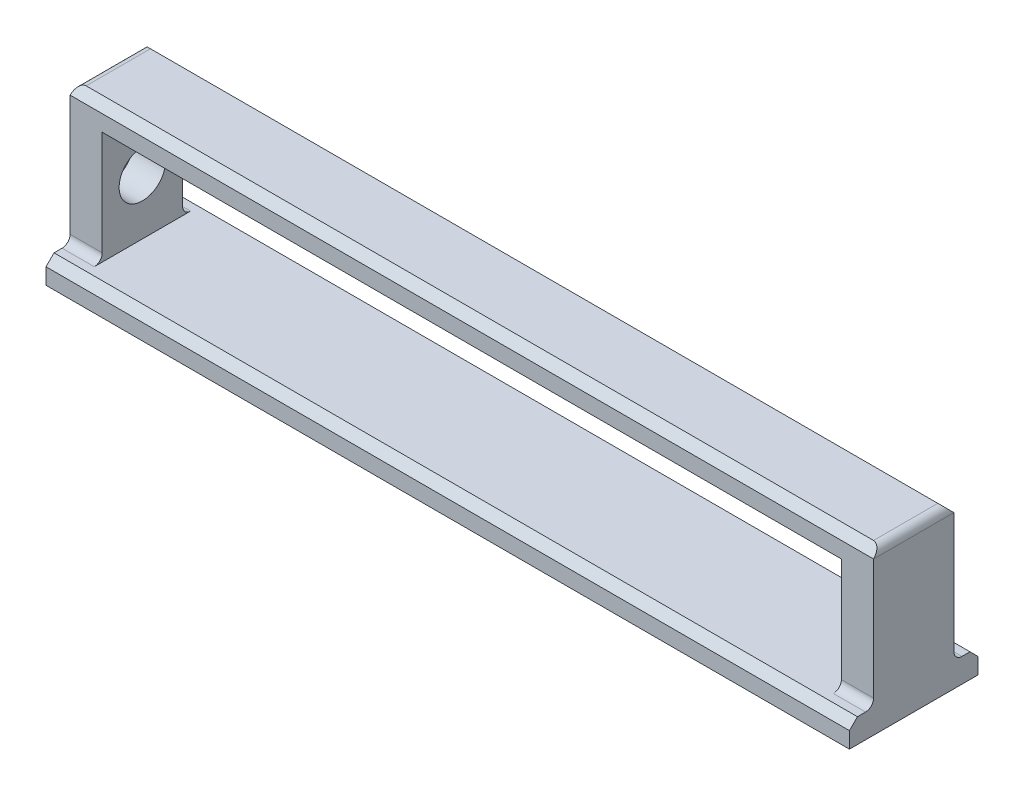
SolidWorks part; units mm, degrees
material "铸造碳钢"
ref_plane "Front Plane" through (0, 0, 0) normal (0, 0, 1) x (1, 0, 0)
ref_plane "Top Plane" through (0, 0, 0) normal (0, 1, 0) x (1, 0, 0)
ref_plane "Right Plane" through (0, 0, 0) normal (1, 0, 0) x (0, 0, -1)
sketch "Sketch1" plane through (0, 0, 0) normal (0, 0, 1) x (1, 0, 0)
  line L0 (0, 1000) -> (5000, 1000)
  line L3 (5000, 0) -> (0, 0)
  line L4 (5000, 1000) -> (5000, 0)
  line L11 (0, 1000) -> (0, 0)
  dimension "D1" = 5000
  dimension "D3" = 1000
extrude "Boss-Extrude1" add sketch "Sketch1" along normal mid plane 500
sketch "Sketch2" plane through (0, 0, 250) normal (0, 0, 1) x (1, 0, 0)
  line L0 (2500, 1000) -> (2500, 0) construction
  line L1 (4800, 850) -> (200, 850)
  line L2 (4800, 850) -> (4800, 150)
  line L3 (4800, 150) -> (200, 150)
  line L4 (200, 850) -> (200, 150)
  line L5 (4800, 850) -> (200, 150) construction
  line L6 (4800, 150) -> (200, 850) construction
  line L7 (5000, 1000) -> (0, 1000) construction
  line L8 (0, 0) -> (5000, 0) construction
  line L9 (5000, 0) -> (5000, 1000) construction
  point P0 (2500, 500)
  dimension "D1" = 200
  dimension "D2" = 150
extrude "Cut-Extrude1" cut sketch "Sketch2" against normal through all
sketch "Sketch3" plane through (0, 0, 0) normal (-1, 0, 0) x (0, 0, 1)
  line L0 (0, 1000) -> (0, 0) construction
  line L1 (250, 1000) -> (-250, 1000) construction
  line L2 (250, 0) -> (-250, 0) construction
  circle A0 centre (0, 500) radius 145
  dimension "D1" = 290
  dimension "D2" = 500
extrude "Cut-Extrude2" cut sketch "Sketch3" against normal up to surface (200 mm away) and the other way through all up to face at (200, 500, 0)
sketch "Sketch4" plane through (0, 0, 0) normal (0, -1, 0) x (1, 0, 0)
  line L0 (2500, 250) -> (2500, -250) construction
  line L1 (0, 250) -> (5000, 250) construction
  line L2 (0, -250) -> (5000, -250) construction
  line L4 (0, 400) -> (5000, 400)
  line L5 (0, 400) -> (0, -400)
  line L6 (0, -400) -> (5000, -400)
  line L7 (5000, 400) -> (5000, -400)
  line L8 (0, 400) -> (5000, -400) construction
  line L9 (0, -400) -> (5000, 400) construction
  point P6 (2500, 0)
  dimension "D1" = 800
extrude "Boss-Extrude2" add sketch "Sketch4" against normal up to surface (150 mm away) up to face at (2500, 150, 0)
sketch "Sketch5" plane through (0, 0, 400) normal (0, 0, 1) x (1, 0, 0)
  line L0 (200, 150) -> (0, 150) construction
  line L1 (0, 0) -> (-1000, 0)
  line L2 (0, 0) -> (0, 150)
  line L3 (0, 150) -> (-1000, 150)
  line L4 (-1000, 0) -> (-1000, 150)
  dimension "D1" = 1000
chamfer "Chamfer1" distance 50 angle 45 4 edges at (2500, 1000, -250) (2500, 1000, 250) (2500, 150, 400) (2500, 150, -400)
fillet "Fillet1" radius 50 4 edges at (100, 150, -250) (100, 150, 250) (4900, 150, 250) (4900, 150, -250)
fillet "Fillet2" radius 50 2 edges at (5000, 1000, 0) (0, 1000, 0)
sketch "Sketch6" plane through (4800, 0, 0) normal (1, 0, 0) x (0, 0, -1)
  circle A0 centre (0, 500) radius 150
  dimension "D1" = 300
extrude "Cut-Extrude3" cut sketch "Sketch6" along normal blind 90
